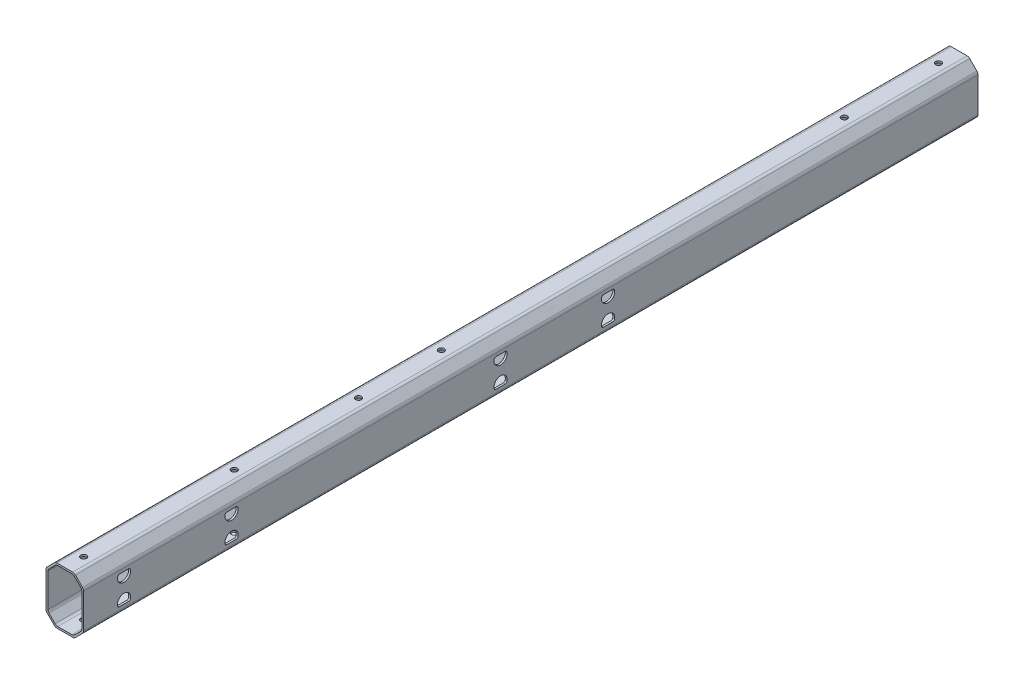
from build123d import *

# Parameters (mm, degrees)
EXTRUDE_1_DEPTH          = 475
FILLET_1_R               = 2
SKETCH_2_R               = 1.55
CUT_EXTRUDE_1_DEPTH      = 477.051467806
CUT_EXTRUDE_2_DEPTH      = 476.657439761
CUT_EXTRUDE_2_DEPTH_BACK = 476.657439761
SKETCH_3_R               = 1.05
CUT_EXTRUDE_START        = -1
SKETCH_4_R               = 1.05
CUT_EXTRUDE_3_DEPTH      = 1
FILLET_2_R               = 1


with BuildPart() as part:
    # 草图1 → 凸台-拉伸1 (new body)
    with BuildSketch(Plane.XY):
        Polygon((-5, 15), (5, 15), (10, 10), (10, -10), (5, -15), (-5, -15), (-10, -10), (-10, 10), align=None)
        Polygon((-9, 9.585786438), (-4.585786438, 14), (4.585786438, 14), (9, 9.585786438), (9, -9.585786438), (4.585786438, -14), (-4.585786438, -14), (-9, -9.585786438), align=None, mode=Mode.SUBTRACT)
    extrude(amount=EXTRUDE_1_DEPTH)

    # 圆角1
    fillet_1_edges = [part.edges().sort_by_distance(p)[0] for p in [
        (-5, 15, 237.5),
        (5, 15, 237.5),
        (10, 10, 237.5),
        (10, -10, 237.5),
        (5, -15, 237.5),
        (-5, -15, 237.5),
        (-10, -10, 237.5),
        (-10, 10, 237.5),
        (-9, 9.585786438, 237.5),
        (-9, -9.585786438, 237.5),
        (-4.585786438, -14, 237.5),
        (4.585786438, -14, 237.5),
        (9, -9.585786438, 237.5),
        (9, 9.585786438, 237.5),
        (4.585786438, 14, 237.5),
        (-4.585786438, 14, 237.5),
    ]]
    fillet(fillet_1_edges, radius=FILLET_1_R)

    # 草图2 → 切除-拉伸1 (cut, through all)
    with BuildSketch(Plane(origin=(0, 15, 0), x_dir=(1, 0, 0), z_dir=(0, 1, 0))):
        with Locations(Location((0, -11, 0), (0, 0, 270))):
            Circle(SKETCH_2_R)
        with Locations(Location((0, -61, 0), (0, 0, 270))):
            Circle(SKETCH_2_R)
        with Locations(Location((0, -385, 0), (0, 0, 270))):
            Circle(SKETCH_2_R)
        with Locations(Location((0, -465, 0), (0, 0, 270))):
            Circle(SKETCH_2_R)
        with Locations(Location((0, -319, 0), (0, 0, 270))):
            Circle(SKETCH_2_R)
        with Locations(Location((0, -275, 0), (0, 0, 270))):
            Circle(SKETCH_2_R)
    extrude(amount=-CUT_EXTRUDE_1_DEPTH, mode=Mode.SUBTRACT)

    # 草图3 → 切除-拉伸2 (cut, two sides: drawn at the far end of the back side and taken through both)
    with BuildSketch(Plane.ZY.offset(10).offset(-CUT_EXTRUDE_2_DEPTH_BACK)):
        with Locations((396.45, 6)):
            Circle(SKETCH_3_R)
        with Locations((396.45, -6)):
            Circle(SKETCH_3_R)
        with Locations((453.55, 6)):
            Circle(SKETCH_3_R)
        with Locations((453.55, -6)):
            Circle(SKETCH_3_R)
        with Locations((196.45, 6)):
            Circle(SKETCH_3_R)
        with Locations((196.45, -6)):
            Circle(SKETCH_3_R)
        with Locations((253.55, 6)):
            Circle(SKETCH_3_R)
        with Locations((253.55, -6)):
            Circle(SKETCH_3_R)
    extrude(amount=CUT_EXTRUDE_2_DEPTH + CUT_EXTRUDE_2_DEPTH_BACK, mode=Mode.SUBTRACT)

    # 草图4 → 切除-拉伸3 (cut)
    # profile 1 of 8: a face of its own
    with BuildSketch(Plane(origin=(10, 0, 0), x_dir=(0, 0, -1), z_dir=(1, 0, 0)).offset(CUT_EXTRUDE_START)):
        with BuildLine():
            Line((-450.38772234, 7.5), (-456.71227766, 7.5))
            ThreePointArc((-456.71227766, 7.5), (-454.318774411, 2.585474278), (-450.05, 6))
            ThreePointArc((-450.05, 6), (-450.135474278, 6.768774411), (-450.38772234, 7.5))
        make_face()
        with Locations(Location((-453.55, 6, 0), (0, 0, 180))):
            Circle(SKETCH_4_R, mode=Mode.SUBTRACT)
    # profile 2 of 8: a face of its own
    with BuildSketch(Plane(origin=(10, 0, 0), x_dir=(0, 0, -1), z_dir=(1, 0, 0)).offset(CUT_EXTRUDE_START)):
        with BuildLine():
            ThreePointArc((-450.05, -6), (-454.318774411, -2.585474278), (-456.71227766, -7.5))
            Line((-456.71227766, -7.5), (-450.38772234, -7.5))
            ThreePointArc((-450.38772234, -7.5), (-450.135474278, -6.768774411), (-450.05, -6))
        make_face()
        with Locations(Location((-453.55, -6, 0), (0, 0, 180))):
            Circle(SKETCH_4_R, mode=Mode.SUBTRACT)
    # profile 3 of 8: a face of its own
    with BuildSketch(Plane(origin=(10, 0, 0), x_dir=(0, 0, -1), z_dir=(1, 0, 0)).offset(CUT_EXTRUDE_START)):
        with BuildLine():
            Line((-399.61227766, -7.5), (-393.28772234, -7.5))
            ThreePointArc((-393.28772234, -7.5), (-393.035474278, -6.768774411), (-392.95, -6))
            ThreePointArc((-392.95, -6), (-397.218774411, -2.585474278), (-399.61227766, -7.5))
        make_face()
        with Locations(Location((-396.45, -6, 0), (0, 0, 180))):
            Circle(SKETCH_4_R, mode=Mode.SUBTRACT)
    # profile 4 of 8: a face of its own
    with BuildSketch(Plane(origin=(10, 0, 0), x_dir=(0, 0, -1), z_dir=(1, 0, 0)).offset(CUT_EXTRUDE_START)):
        with BuildLine():
            ThreePointArc((-392.95, 6), (-393.035474278, 6.768774411), (-393.28772234, 7.5))
            Line((-393.28772234, 7.5), (-399.61227766, 7.5))
            ThreePointArc((-399.61227766, 7.5), (-397.218774411, 2.585474278), (-392.95, 6))
        make_face()
        with Locations(Location((-396.45, 6, 0), (0, 0, 180))):
            Circle(SKETCH_4_R, mode=Mode.SUBTRACT)
    # profile 5 of 8: a face of its own
    with BuildSketch(Plane(origin=(10, 0, 0), x_dir=(0, 0, -1), z_dir=(1, 0, 0)).offset(CUT_EXTRUDE_START)):
        with BuildLine():
            Line((-250.38772234, 7.5), (-256.71227766, 7.5))
            ThreePointArc((-256.71227766, 7.5), (-254.318774411, 2.585474278), (-250.05, 6))
            ThreePointArc((-250.05, 6), (-250.135474278, 6.768774411), (-250.38772234, 7.5))
        make_face()
        with Locations(Location((-253.55, 6, 0), (0, 0, 180))):
            Circle(SKETCH_4_R, mode=Mode.SUBTRACT)
    # profile 6 of 8: a face of its own
    with BuildSketch(Plane(origin=(10, 0, 0), x_dir=(0, 0, -1), z_dir=(1, 0, 0)).offset(CUT_EXTRUDE_START)):
        with BuildLine():
            ThreePointArc((-250.05, -6), (-254.318774411, -2.585474278), (-256.71227766, -7.5))
            Line((-256.71227766, -7.5), (-250.38772234, -7.5))
            ThreePointArc((-250.38772234, -7.5), (-250.135474278, -6.768774411), (-250.05, -6))
        make_face()
        with Locations(Location((-253.55, -6, 0), (0, 0, 180))):
            Circle(SKETCH_4_R, mode=Mode.SUBTRACT)
    # profile 7 of 8: a face of its own
    with BuildSketch(Plane(origin=(10, 0, 0), x_dir=(0, 0, -1), z_dir=(1, 0, 0)).offset(CUT_EXTRUDE_START)):
        with BuildLine():
            ThreePointArc((-192.95, 6), (-193.035474278, 6.768774411), (-193.28772234, 7.5))
            Line((-193.28772234, 7.5), (-199.61227766, 7.5))
            ThreePointArc((-199.61227766, 7.5), (-197.218774411, 2.585474278), (-192.95, 6))
        make_face()
        with Locations(Location((-196.45, 6, 0), (0, 0, 180))):
            Circle(SKETCH_4_R, mode=Mode.SUBTRACT)
    # profile 8 of 8: a face of its own
    with BuildSketch(Plane(origin=(10, 0, 0), x_dir=(0, 0, -1), z_dir=(1, 0, 0)).offset(CUT_EXTRUDE_START)):
        with BuildLine():
            Line((-199.61227766, -7.5), (-193.28772234, -7.5))
            ThreePointArc((-193.28772234, -7.5), (-193.035474278, -6.768774411), (-192.95, -6))
            ThreePointArc((-192.95, -6), (-197.218774411, -2.585474278), (-199.61227766, -7.5))
        make_face()
        with Locations(Location((-196.45, -6, 0), (0, 0, 180))):
            Circle(SKETCH_4_R, mode=Mode.SUBTRACT)
    extrude(amount=CUT_EXTRUDE_3_DEPTH, mode=Mode.SUBTRACT)

    # 圆角2
    fillet_2_edges = [part.edges().sort_by_distance(p)[0] for p in [
        (9.5, -7.5, 456.71227766),
        (9.5, -7.5, 450.38772234),
        (9.5, -7.5, 393.28772234),
        (9.5, -7.5, 399.61227766),
        (9.5, 7.5, 399.61227766),
        (9.5, 7.5, 393.28772234),
        (9.5, 7.5, 250.38772234),
        (9.5, 7.5, 256.71227766),
        (9.5, -7.5, 193.28772234),
        (9.5, -7.5, 199.61227766),
        (9.5, 7.5, 199.61227766),
        (9.5, 7.5, 193.28772234),
        (9.5, -7.5, 256.71227766),
        (9.5, -7.5, 250.38772234),
        (9.5, 7.5, 450.38772234),
        (9.5, 7.5, 456.71227766),
    ]]
    fillet(fillet_2_edges, radius=FILLET_2_R)


solid = part.part
